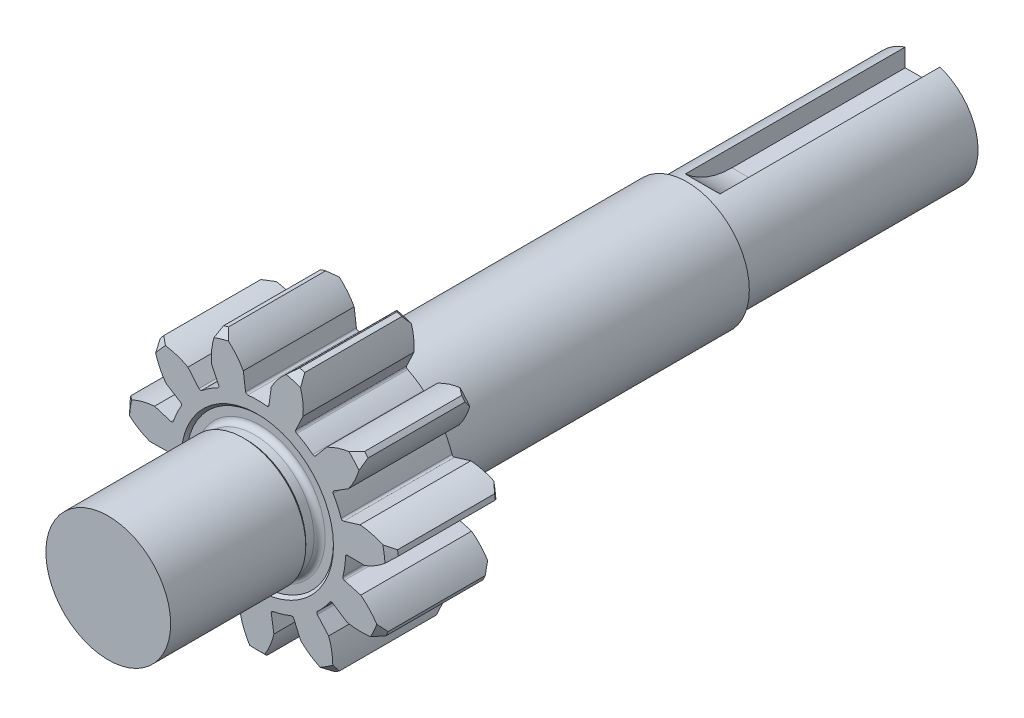
from build123d import *

# Parameters (mm, degrees)
CIRCLE_R                 = 19.5
BLANK_DEPTH              = 8
TOOTH_CHAMFER_SIZE       = 1
GEAR_SHAPING_DEPTH       = 8
FILLET2_R                = 0.3
CIRPATTERN2_COUNT        = 11
FILLET2_OF_CIRPATTERN2_R = 0.3
SKETCH1_R                = 9
BOSS_EXTRUDE1_DEPTH      = 21.5
BOSS_EXTRUDE2_START      = -117.5
SKETCH2_R                = 8
BOSS_EXTRUDE2_DEPTH      = 34
SKETCH3_R                = 9
BOSS_EXTRUDE3_DEPTH      = 46
CUT_EXTRUDE1_DEPTH       = 2.5
FILLET3_R                = 0.8


with BuildPart() as part:
    # Circle → Blank (new, symmetric)
    with BuildSketch(Plane.XY):
        Circle(CIRCLE_R)
    extrude(amount=BLANK_DEPTH, both=True)

    # Tooth chamfer
    tooth_chamfer_edges = [part.edges().sort_by_distance(p)[0] for p in [
        (-19.5, 0, -8),
        (-19.5, 0, 8),
    ]]
    chamfer(tooth_chamfer_edges, length=TOOTH_CHAMFER_SIZE)

    # Tooth profile → Gear shaping (cut, symmetric)
    with BuildSketch(Plane.XY):
        with BuildLine():
            ThreePointArc((-1.657319875, 12.641827037), (0, 12.75), (1.657319875, 12.641827037))
            Line((1.657319875, 12.641827037), (2.015421626, 15.373382045))
            add(Edge.make_bspline(
                [(2.015421626, 15.373382045), (2.101128121, 15.535173288), (2.381258182, 16.022451997), (2.940334149, 16.812235008), (3.736790612, 17.674048579), (4.482655711, 18.321814632), (4.965077907, 18.691820635), (5.129920603, 18.813131441)],
                knots=[0.02088102, 0.02088102, 0.02088102, 0.02088102, 0.02088102, 0.029959916, 0.048733667, 0.068727063, 0.078876106, 0.078876106, 0.078876106, 0.078876106, 0.078876106], degree=4))
            ThreePointArc((5.129920603, 18.813131441), (0, 19.5), (-5.129920604, 18.813131441))
            add(Edge.make_bspline(
                [(-2.015421626, 15.373382045), (-2.101128121, 15.535173287), (-2.381258181, 16.022451997), (-2.940334148, 16.812235007), (-3.736790612, 17.674048577), (-4.482655711, 18.321814631), (-4.965077907, 18.691820635), (-5.129920604, 18.813131441)],
                knots=[0.02088102, 0.02088102, 0.02088102, 0.02088102, 0.02088102, 0.029959916, 0.048733667, 0.068727063, 0.078876106, 0.078876106, 0.078876106, 0.078876106, 0.078876106], degree=4))
            Line((-2.015421626, 15.373382045), (-1.657319875, 12.641827037))
        make_face()
    gear_shaping = extrude(amount=GEAR_SHAPING_DEPTH, both=True, mode=Mode.SUBTRACT)

    # Fillet2
    fillet2_edges = [part.edges().sort_by_distance(p)[0] for p in [
        (1.657319875, 12.641827037, 0),
        (-1.657319875, 12.641827037, 0),
    ]]
    fillet(fillet2_edges, radius=FILLET2_R)

    # CirPattern2: Gear shaping ×11 about axis
    cirpattern2_axis = Axis((0, 0, 8), (0, 0, -1))
    for i in range(1, CIRPATTERN2_COUNT):
        add(gear_shaping.rotate(cirpattern2_axis, i * 360 / CIRPATTERN2_COUNT), mode=Mode.SUBTRACT)

    # Fillet2 of CirPattern2
    fillet2_of_cirpattern2_edges = [part.edges().sort_by_distance(p)[0] for p in [
        (8.228913903, 9.738966885, 0),
        (5.440461504, 11.530996428, 0),
        (12.18788591, 3.744053559, 0),
        (10.810934795, 6.759155927, 0),
        (12.277290256, -3.439570318, 0),
        (12.749012676, -0.158668822, 0),
        (8.468741693, -9.531154922, 0),
        (10.639369112, -7.026117342, 0),
        (1.97142748, -12.596665181, 0),
        (5.151801029, -11.66282325, 0),
        (-5.151801029, -11.66282325, 0),
        (-1.97142748, -12.596665181, 0),
        (-10.639369112, -7.026117342, 0),
        (-8.468741693, -9.531154922, 0),
        (-12.749012676, -0.158668822, 0),
        (-12.277290256, -3.439570318, 0),
        (-10.810934795, 6.759155927, 0),
        (-12.18788591, 3.744053559, 0),
        (-5.440461504, 11.530996428, 0),
        (-8.228913903, 9.738966885, 0),
    ]]
    fillet(fillet2_of_cirpattern2_edges, radius=FILLET2_OF_CIRPATTERN2_R)

    # Sketch1 → Boss-Extrude1 (add)
    with BuildSketch(Plane.XY.offset(8)):
        Circle(SKETCH1_R)
    extrude(amount=BOSS_EXTRUDE1_DEPTH)



with BuildPart() as body_2:
    # Sketch2 → Boss-Extrude2 (new body)
    with BuildSketch(Plane.XY.offset(29.5).offset(BOSS_EXTRUDE2_START)):
        Circle(SKETCH2_R)
    extrude(amount=BOSS_EXTRUDE2_DEPTH)


with BuildPart() as part_1:
    add(part.part)

    add(body_2.part)  # Boss-Extrude3 merges body 2
    # Sketch3 → Boss-Extrude3 (add)
    with BuildSketch(Plane.XY.offset(-54)):
        Circle(SKETCH3_R)
    extrude(amount=BOSS_EXTRUDE3_DEPTH)

    # Sketch4 → Cut-Extrude1 (cut, symmetric)
    with BuildSketch(Plane(origin=(0, 0, 0), x_dir=(0, 0, -1), z_dir=(1, 0, 0))):
        with BuildLine():
            Line((88, 5), (63, 5))
            ThreePointArc((63, 5), (59.127016654, 5.780455543), (55.858571571, 8))
            Line((55.858571571, 8), (88, 8))
            Line((88, 8), (88, 5))
        make_face()
    extrude(amount=CUT_EXTRUDE1_DEPTH, both=True, mode=Mode.SUBTRACT)

    # Sketch5 → Cut-Revolve1 (revolve, cut)
    with BuildSketch(Plane(origin=(0, 0, 0), x_dir=(0, 0, -1), z_dir=(1, 0, 0)), mode=Mode.PRIVATE) as cut_revolve1_sk:
        Polygon((8, 11), (7.6, 10.6), (7.6, 8.6), (9.6, 8.6), (10, 9), (8, 9), align=None)
        Polygon((-8, 9), (-8, 11), (-7.6, 10.6), (-7.6, 8.6), (-9.6, 8.6), (-10, 9), align=None)
    revolve(cut_revolve1_sk.sketch.rotate(Axis((0, 0, 0), (0, 0, -1)), 90), axis=Axis((0, 0, 0), (0, 0, -1)), mode=Mode.SUBTRACT)

    # Fillet3
    fillet3_edges = [part_1.edges().sort_by_distance(p)[0] for p in [
        (-8.6, 0, -7.6),
        (-8.6, 0, 7.6),
    ]]
    fillet(fillet3_edges, radius=FILLET3_R)


solid = part_1.part
